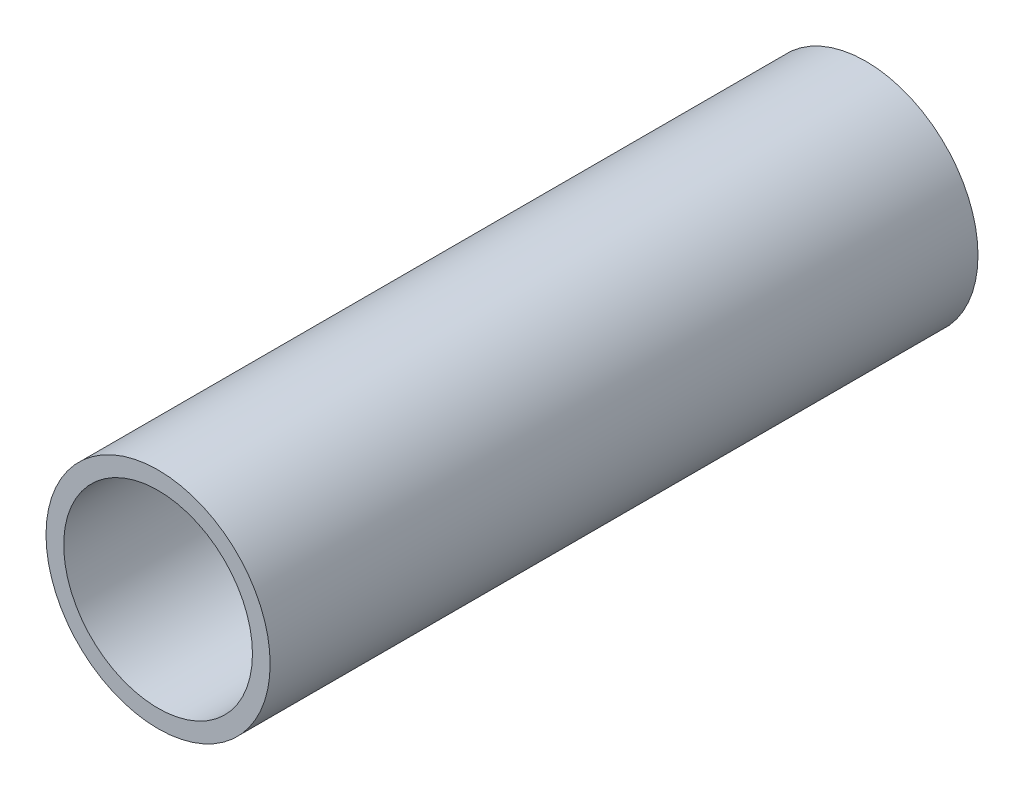
from build123d import *

# Parameters (mm, degrees)
SKETCH1_R           = 2.413
SKETCH1_R_2         = 2.032
BOSS_EXTRUDE1_DEPTH = 15.24
SCALE1_SCALE        = 2


with BuildPart() as part:
    # Sketch1 → Boss-Extrude1 (new body)
    with BuildSketch(Plane.XY):
        Circle(SKETCH1_R)
        Circle(SKETCH1_R_2, mode=Mode.SUBTRACT)
    extrude(amount=-BOSS_EXTRUDE1_DEPTH)


with BuildPart() as part_1:
    # Scale1: scaled about (0, 0, 0)
    add(part.part.scale(SCALE1_SCALE))


solid = part_1.part
